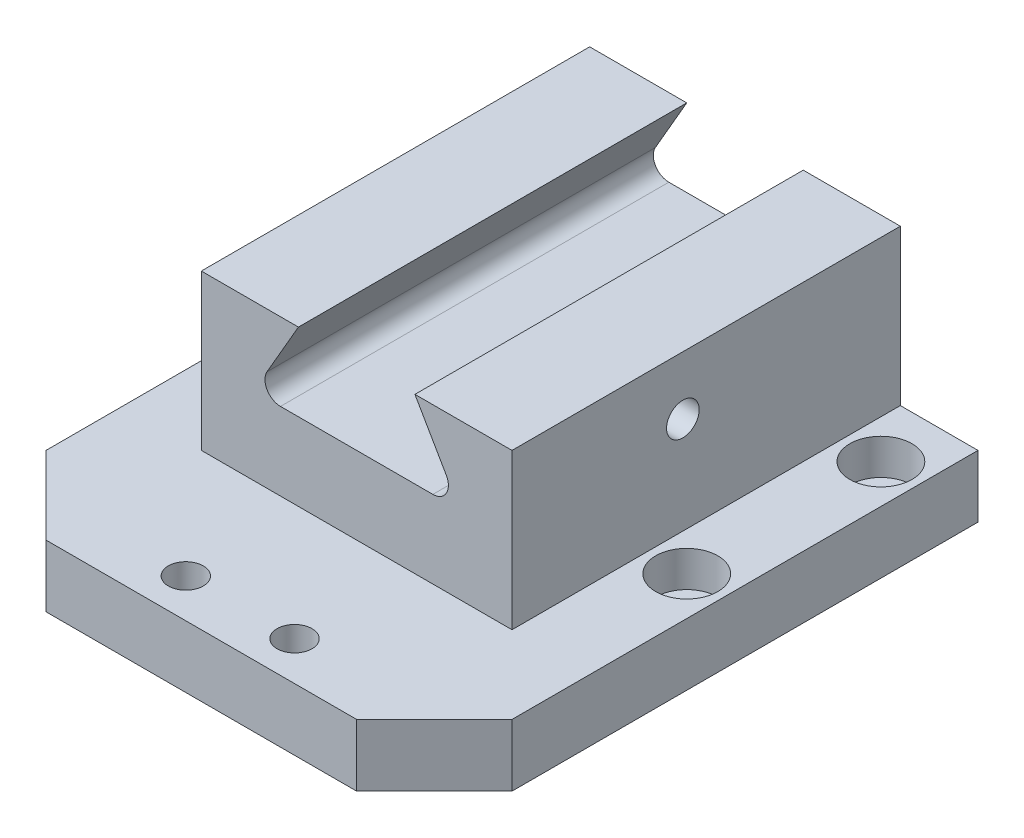
SolidWorks part; units mm, degrees
ref_plane "Front Plane" through (0, 0, 0) normal (0, 0, 1) x (1, 0, 0)
ref_plane "Top Plane" through (0, 0, 0) normal (0, 1, 0) x (1, 0, 0)
ref_plane "Right Plane" through (0, 0, 0) normal (1, 0, 0) x (0, 0, -1)
sketch "Sketch1" plane through (0, 0, 0) normal (0, 0, 1) x (1, 0, 0)
  line L1 (-20, 10) -> (20, 10)
  line L2 (-20, 10) -> (-20, -10)
  line L3 (-20, -10) -> (20, -10)
  line L4 (20, 10) -> (20, -10)
  line L5 (-20, 10) -> (20, -10) construction
  line L6 (-20, -10) -> (20, 10) construction
  point P0 (0, 0)
  dimension "D1" = 20
  dimension "D2" = 40
extrude "Boss-Extrude1" add sketch "Sketch1" along normal mid plane 50
sketch "Sketch2" plane through (0, -10, 0) normal (0, -1, 0) x (1, 0, 0)
  line L0 (-20, -25) -> (20, -25) construction
  line L1 (30, -25) -> (-30, -25)
  line L2 (30, -25) -> (30, 45)
  line L3 (30, 45) -> (-30, 45)
  line L4 (-30, -25) -> (-30, 45)
  line L5 (30, -25) -> (-30, 45) construction
  line L6 (30, 45) -> (-30, -25) construction
  dimension "D1" = 70
  dimension "D2" = 60
  dimension "D3" = 30
extrude "Boss-Extrude2" add sketch "Sketch2" along normal blind 8
sketch "Sketch3" plane through (0, 0, 25) normal (0, 0, 1) x (1, 0, 0)
  line L0 (0, 10) -> (0, 0) construction
  line L1 (20, 10) -> (-20, 10) construction
  line L2 (-7.5, 10) -> (-11.5415, 3)
  line L3 (-9.8094, 0) -> (9.8094, 0)
  line L4 (11.5415, 3) -> (7.5, 10)
  line L5 (-7.5, 10) -> (7.5, 10)
  arc A0 (9.8094, 0) -> (11.5415, 3) centre (9.8094, 2) ccw
  arc A1 (-11.5415, 3) -> (-9.8094, 0) centre (-9.8094, 2) ccw
  dimension "D4" = 2
  dimension "D1" = 60
  dimension "D2" = 15
  dimension "D3" = 10
extrude "Cut-Extrude1" cut sketch "Sketch3" against normal through all
chamfer "Chamfer1" distance 10 angle 45 2 edges at (30, -14, 45) (-30, -14, 45)
hole_wizard "Hole Size per Socket Head Cap Screw Type1" positions "Sketch7" profile "Sketch6" counterbore size "M4" standard "GB" end condition through all
sketch "Sketch7" plane through (0, -18, 0) normal (0, -1, 0) x (1, 0, 0)
  point P1 (7, 40)
  point P4 (-7, 40)
sketch "Sketch6" plane through (7, -18, 40) normal (1, 0, 0) x (0, 0, -1)
  line L0 (0, 0) -> (0, 28)
  line L1 (0, 28) -> (2.25, 28)
  line L3 (2.25, 28) -> (2.25, 4.6)
  line L4 (2.25, 4.6) -> (4, 4.6)
  line L5 (4, 4.6) -> (4, 0)
  line L7 (4, 0) -> (0, 0)
  line L11 (0, -6.35) -> (0, 107.95) construction
  dimension "通孔孔直径" = 4.5
  dimension "通孔孔深度" = 28
  dimension "柱形沉头孔直径" = 8
  dimension "柱形沉头孔深度" = 4.6
hole_wizard "Hole Size per Socket Head Cap Screw Type2" positions "Sketch9" profile "Sketch8" counterbore size "M4" standard "GB" end condition through all
sketch "Sketch9" plane through (0, -10, 0) normal (0, 1, 0) x (-1, 0, 0)
  line L0 (0, -25) -> (0, 45) construction
  line L1 (9.8094, -25) -> (-9.8094, -25) construction
  line L2 (-20, 45) -> (20, 45) construction
  line L6 (30, -25) -> (20, -25) construction
  point P1 (25, -17.5)
  point P3 (25, 7.5)
  point P5 (-25, -17.5)
  point P7 (-25, 7.5)
  dimension "D1" = 50
  dimension "D2" = 25
  dimension "D3" = 7.5
sketch "Sketch8" plane through (-25, -10, -17.5) normal (1, 0, 0) x (0, 0, 1)
  line L0 (0, 0) -> (0, 8)
  line L1 (0, 8) -> (2.25, 8)
  line L3 (2.25, 8) -> (2.25, 4.6)
  line L4 (2.25, 4.6) -> (4, 4.6)
  line L5 (4, 4.6) -> (4, 0)
  line L7 (4, 0) -> (0, 0)
  line L11 (0, -6.35) -> (0, 107.95) construction
  dimension "通孔孔直径" = 4.5
  dimension "通孔孔深度" = 8
  dimension "柱形沉头孔直径" = 8
  dimension "柱形沉头孔深度" = 4.6
hole_wizard "M5 Tapped Hole1" positions "Sketch11" profile "Sketch10" tap size "M5" standard "GB"
sketch "Sketch11" plane through (20, 0, 0) normal (1, 0, 0) x (0, 0, -1)
  line L0 (-25, -10) -> (-25, 10) construction
  line L1 (-25, 10) -> (25, 10) construction
  point P0 (-3, 2.5)
  dimension "D1" = 22
  dimension "D2" = 7.5
sketch "Sketch10" plane through (20, 2.5, 3) normal (0, 1, 0) x (0, 0, -1)
  line L0 (0, 0) -> (0, 13.6618)
  line L1 (0, 13.6618) -> (2.1, 12.4)
  line L2 (2.1, 12.4) -> (2.1, 0)
  line L5 (2.1, 0) -> (0, 0)
  line L10 (0, 13.6618) -> (-2.1, 12.4) construction
  line L11 (0, -6.35) -> (0, 107.95) construction
  dimension "螺纹孔钻头直径" = 4.2
  dimension "螺纹孔钻头深度" = 12.4
  dimension "导头角度" = 118
cosmetic thread "Cosmetic Thread1"
hole_wizard "M3 Tapped Hole1" positions "Sketch13" profile "Sketch12" tap size "M3" standard "GB"
sketch "Sketch13" plane through (0, 0, -25) normal (0, 0, -1) x (-1, 0, 0)
  point P1 (14, 5)
  point P4 (-14, 5)
sketch "Sketch12" plane through (-14, 5, -25) normal (1, 0, 0) x (0, 1, 0)
  line L0 (0, 0) -> (0, 8.2511)
  line L1 (0, 8.2511) -> (1.25, 7.5)
  line L2 (1.25, 7.5) -> (1.25, 0)
  line L5 (1.25, 0) -> (0, 0)
  line L10 (0, 8.2511) -> (-1.25, 7.5) construction
  line L11 (0, -6.35) -> (0, 107.95) construction
  dimension "螺纹孔钻头直径" = 2.5
  dimension "螺纹孔钻头深度" = 7.5
  dimension "导头角度" = 118
cosmetic thread "Cosmetic Thread2"
cosmetic thread "Cosmetic Thread3"
